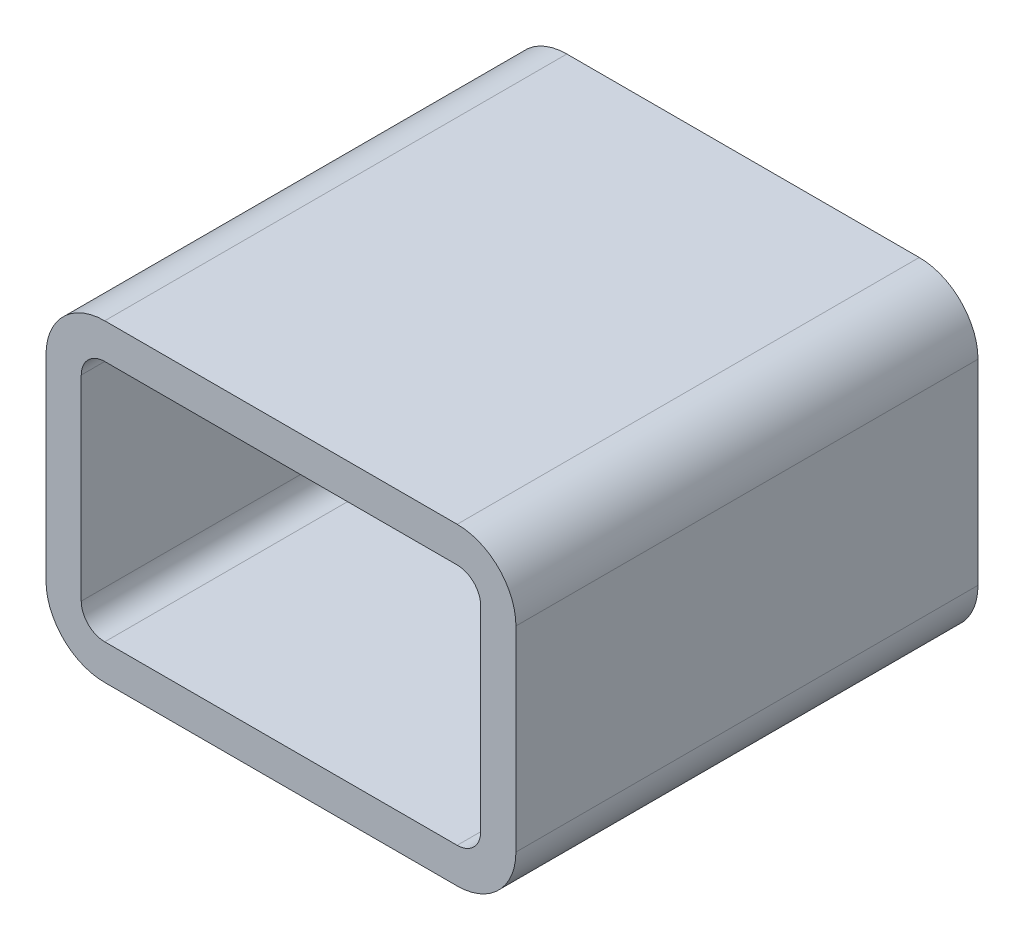
from build123d import *

# Parameters (mm, degrees)
SKETCH_1_W      = 120
SKETCH_1_H      = 80
SKETCH_1_W_2    = 102
SKETCH_1_H_2    = 62
EXTRUDE_1_DEPTH = 118
FILLET_1_R      = 15
FILLET_2_R      = 6


with BuildPart() as part:
    # 草图1 → 凸台-拉伸1 (new body)
    with BuildSketch(Plane.XY):
        Rectangle(SKETCH_1_W, SKETCH_1_H)
        Rectangle(SKETCH_1_W_2, SKETCH_1_H_2, mode=Mode.SUBTRACT)
    extrude(amount=EXTRUDE_1_DEPTH)

    # 圆角1
    fillet_1_edges = [part.edges().sort_by_distance(p)[0] for p in [
        (-60, 40, 59),
        (60, 40, 59),
        (60, -40, 59),
        (-60, -40, 59),
    ]]
    fillet(fillet_1_edges, radius=FILLET_1_R)

    # 圆角2
    fillet_2_edges = [part.edges().sort_by_distance(p)[0] for p in [
        (-51, 31, 59),
        (-51, -31, 59),
        (51, -31, 59),
        (51, 31, 59),
    ]]
    fillet(fillet_2_edges, radius=FILLET_2_R)


solid = part.part
